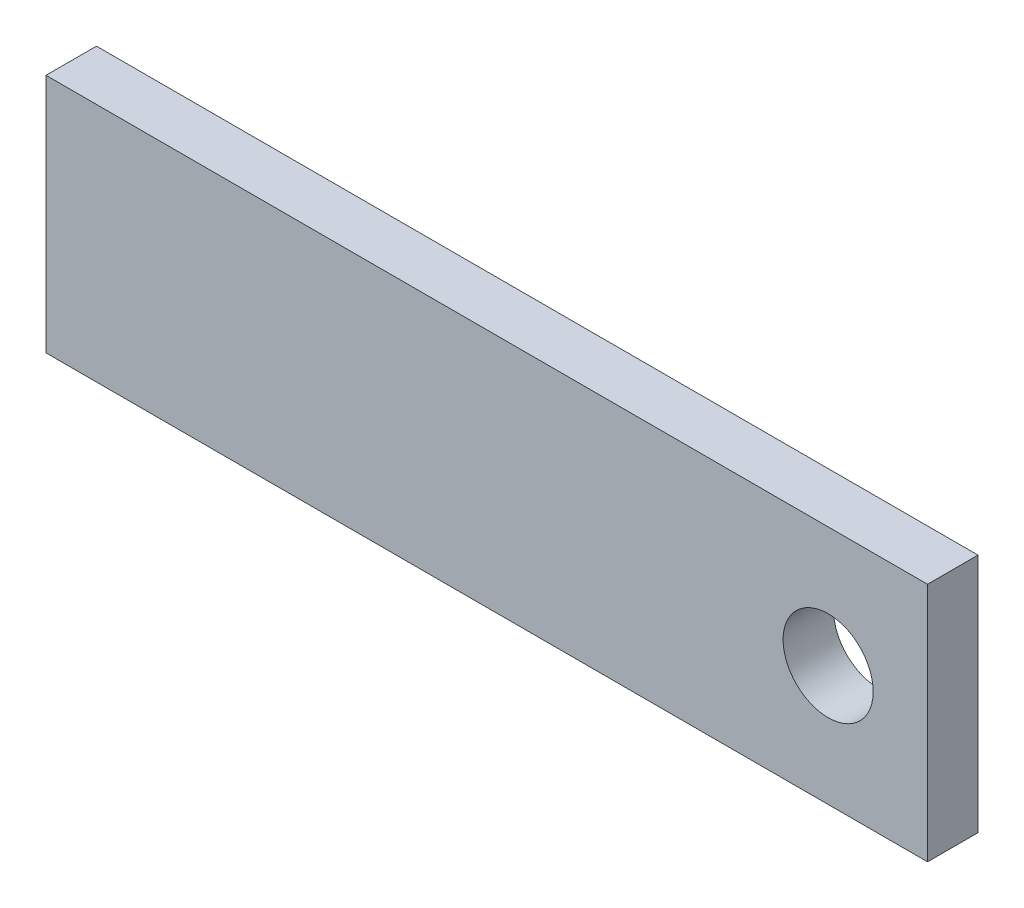
from build123d import *

# Parameters (mm, degrees)
SKETCH1_W           = 139.7
SKETCH1_H           = 38.1
SKETCH1_R           = 7.1374
BOSS_EXTRUDE1_DEPTH = 4


with BuildPart() as part:
    # Sketch1 → Boss-Extrude1 (new, symmetric)
    with BuildSketch(Plane.XY):
        with Locations((-54.102, 0)):
            Rectangle(SKETCH1_W, SKETCH1_H)
        Circle(SKETCH1_R, mode=Mode.SUBTRACT)
    extrude(amount=BOSS_EXTRUDE1_DEPTH, both=True)


solid = part.part
